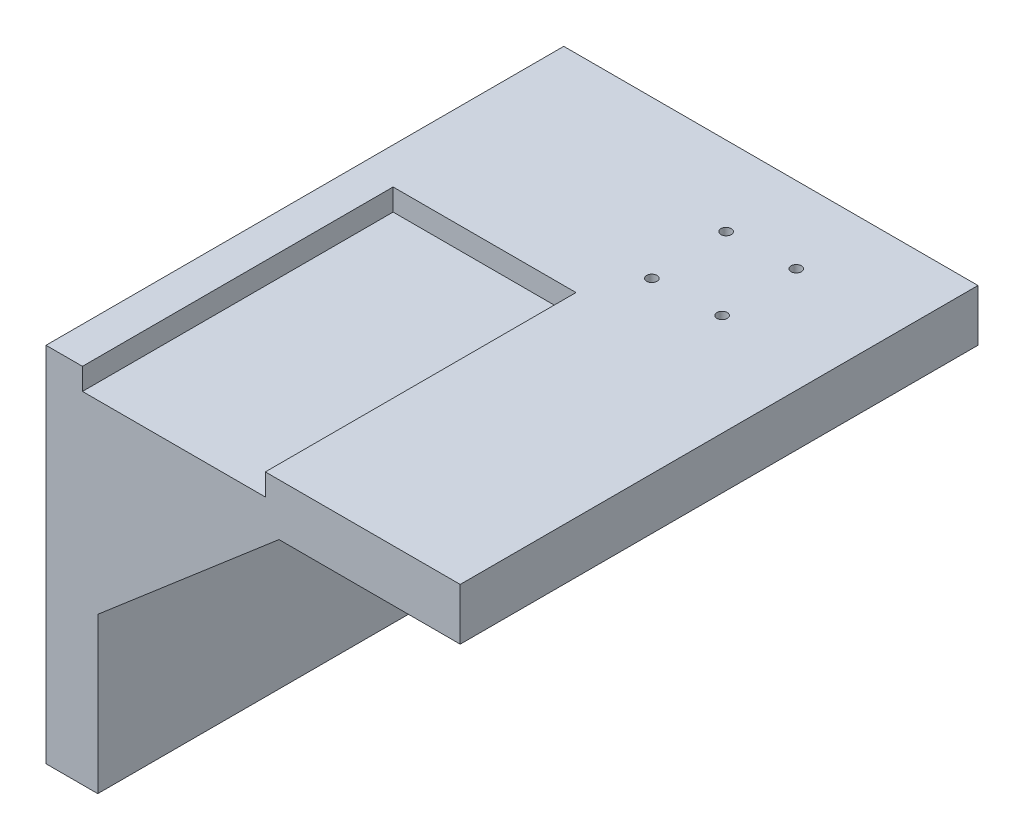
from build123d import *

# Parameters (mm, degrees)
EXTRUDE_1_DEPTH     = 100
SKETCH_2_W          = 35.317953013
SKETCH_2_H          = 4.2
CUT_EXTRUDE_1_DEPTH = 60
RIB_6_REACH         = 112.526
SKETCH_5_WALL_W     = 269.149287264
SKETCH_5_WALL_H     = 10
SKETCH_6_R          = 3
CUT_EXTRUDE_2_DEPTH = 10
SKETCH_7_R          = 1
CUT_EXTRUDE_3_DEPTH = 15


with BuildPart() as part:
    # 草图1 → 凸台-拉伸1 (new body)
    with BuildSketch(Plane.XY):
        Polygon((-37.5, 32.788461538), (42.5, 32.788461538), (42.5, 22.788461538), (-27.5, 22.788461538), (-27.5, -37.211538462), (-37.5, -37.211538462), align=None)
    extrude(amount=EXTRUDE_1_DEPTH)

    # 草图2 → 切除-拉伸1 (cut)
    with BuildSketch(Plane.XY.offset(100)):
        with Locations((-12.799064643, 30.688461538)):
            Rectangle(SKETCH_2_W, SKETCH_2_H)
    extrude(amount=-CUT_EXTRUDE_1_DEPTH, mode=Mode.SUBTRACT)

    # 草图5 wall → 筋6 (add, up to next)
    with BuildSketch(Plane(origin=(-10, 7.788461538, 95), x_dir=(-0.759256602365, -0.650791373456, 0), z_dir=(0.650791373456, -0.759256602365, 0)), mode=Mode.PRIVATE) as rib_6_sk1:
        Rectangle(SKETCH_5_WALL_W, SKETCH_5_WALL_H)
    rib_6_tool1 = extrude(rib_6_sk1.sketch, amount=-RIB_6_REACH, mode=Mode.PRIVATE) - part.part
    add(rib_6_tool1.solids().sort_by_distance((-10, 7.788461538, 95))[0])

    # 草图6 → 切除-拉伸2 (cut)
    with BuildSketch(Plane(origin=(-27.5, 891.532711259, -866.3577183), x_dir=(0, 0, 1), z_dir=(1, 0, 0))):
        with Locations(Location((900.249826396, 880.97002325, 0), (0, 0, 270))):
            Circle(SKETCH_6_R)
        with Locations(Location((890.712774703, 880.97002325, 0), (0, 0, 270))):
            Circle(SKETCH_6_R)
        with Locations(Location((900.249826396, 913.137579673, 0), (0, 0, 270))):
            Circle(SKETCH_6_R)
        with Locations(Location((890.712774703, 913.137579673, 0), (0, 0, 270))):
            Circle(SKETCH_6_R)
    extrude(amount=-CUT_EXTRUDE_2_DEPTH, mode=Mode.SUBTRACT)

    # 草图7 → 切除-拉伸3 (cut)
    with BuildSketch(Plane(origin=(1081.455900364, 22.788461538, -866.3577183), x_dir=(-0.07845909572783148, 0, 0.9969173337331291), z_dir=(0, -1, 0))):
        with Locations(Location((963.085867609, 999.8129825, 0), (0, 0, 265.5))):
            Circle(SKETCH_7_R)
        with Locations(Location((977.974059883, 997.984942349, 0), (0, 0, 265.5))):
            Circle(SKETCH_7_R)
        with Locations(Location((961.501566145, 986.909882529, 0), (0, 0, 265.5))):
            Circle(SKETCH_7_R)
        with Locations(Location((976.389758419, 985.081842378, 0), (0, 0, 265.5))):
            Circle(SKETCH_7_R)
    extrude(amount=-CUT_EXTRUDE_3_DEPTH, mode=Mode.SUBTRACT)


solid = part.part
